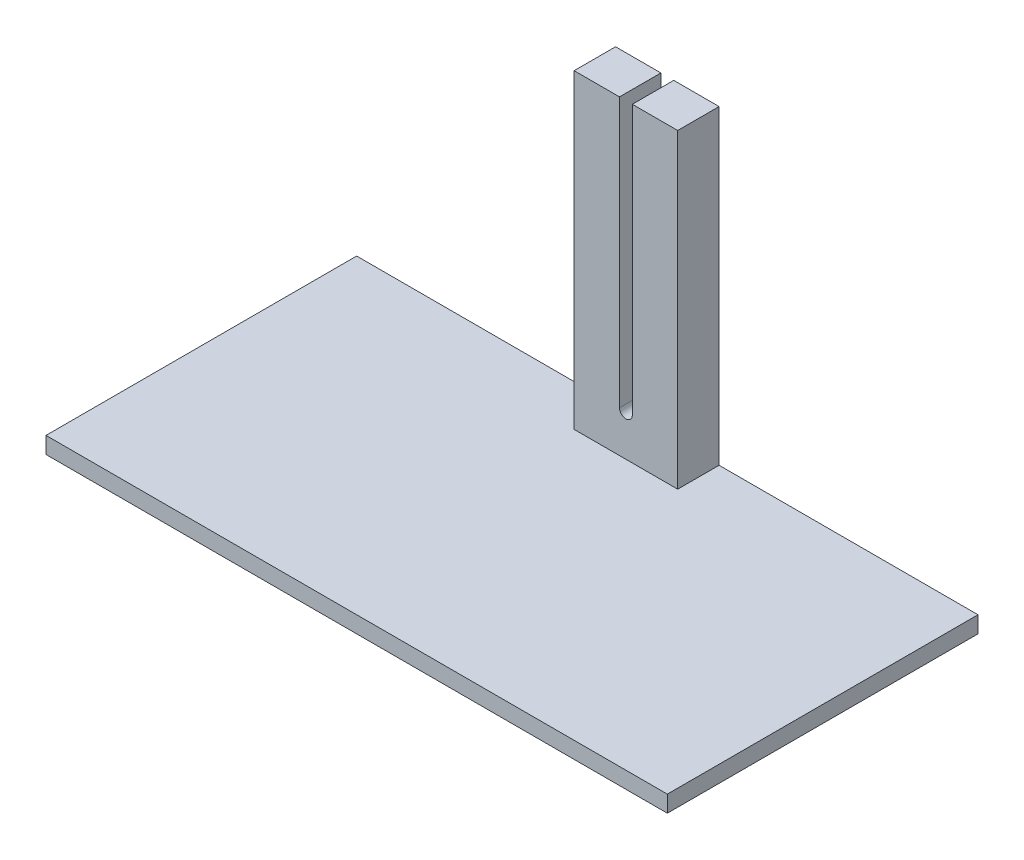
SolidWorks part; units mm, degrees
ref_plane "Front Plane" through (0, 0, 0) normal (0, 0, 1) x (1, 0, 0)
ref_plane "Top Plane" through (0, 0, 0) normal (0, 1, 0) x (1, 0, 0)
ref_plane "Right Plane" through (0, 0, 0) normal (1, 0, 0) x (0, 0, -1)
sketch "Sketch1" plane through (0, 0, 0) normal (0, 1, 0) x (1, 0, 0)
  line L1 (-150, -75) -> (150, -75)
  line L2 (-150, -75) -> (-150, 75)
  line L3 (-150, 75) -> (150, 75)
  line L4 (150, -75) -> (150, 75)
  line L5 (-150, -75) -> (150, 75) construction
  line L6 (-150, 75) -> (150, -75) construction
  point P0 (0, 0)
  dimension "D1" = 300
  dimension "D2" = 150
extrude "Boss-Extrude1" add sketch "Sketch1" along normal blind 8
sketch "Sketch2" plane through (0, 8, 0) normal (0, 1, 0) x (1, 0, 0)
  line L0 (150, 75) -> (-150, 75) construction
  line L1 (-25, 75) -> (25, 75)
  line L2 (-25, 75) -> (-25, 55)
  line L3 (-25, 55) -> (25, 55)
  line L4 (25, 75) -> (25, 55)
  line L5 (-150, 75) -> (-150, -75) construction
  dimension "D1" = 50
  dimension "D2" = 20
  dimension "D3" = 125
extrude "Boss-Extrude2" add sketch "Sketch2" along normal blind 150
sketch "Sketch3" plane through (0, 0, -55) normal (0, 0, 1) x (1, 0, 0)
  line L0 (0, 158) -> (0, 28) construction
  line L1 (-25, 158) -> (25, 158) construction
  line L2 (3.1, 158) -> (3.1, 28)
  line L3 (-3.1, 158) -> (-3.1, 28)
  arc A0 (3.1, 158) -> (-3.1, 158) centre (0, 158) ccw
  arc A1 (-3.1, 28) -> (3.1, 28) centre (0, 28) ccw
  point P5 (0, 93)
  dimension "D1" = 3.1
  dimension "D2" = 130
extrude "Cut-Extrude1" cut sketch "Sketch3" against normal through all
